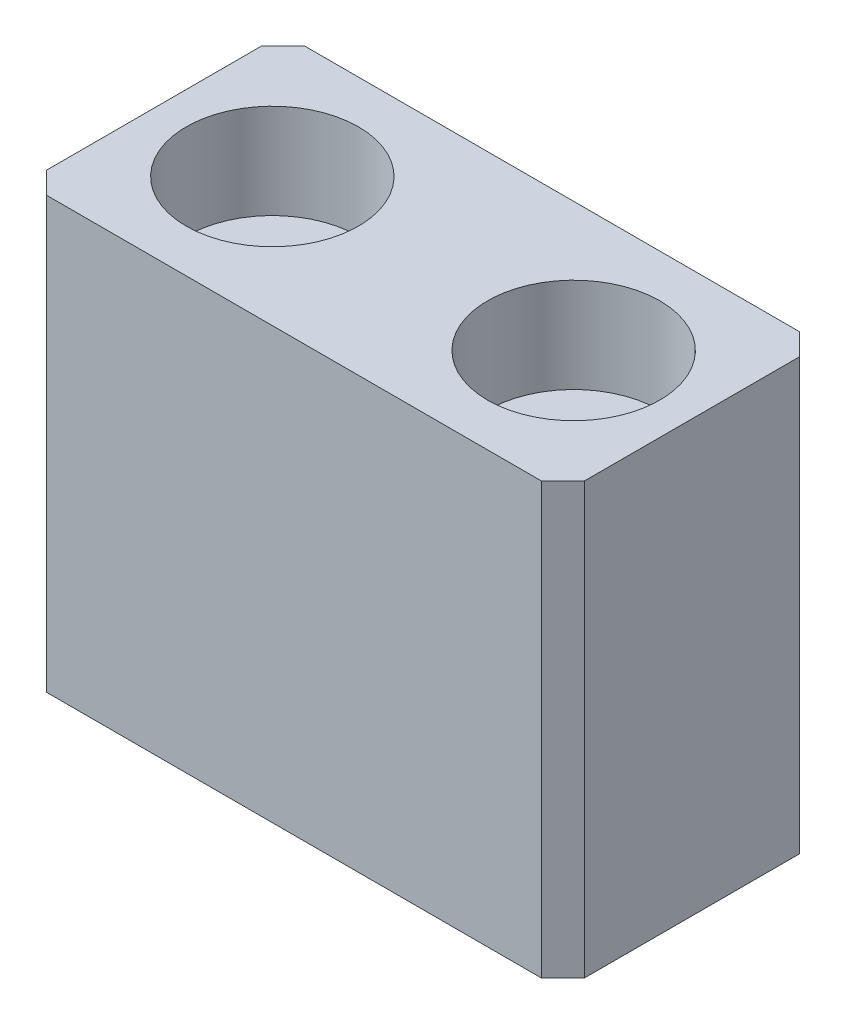
SolidWorks part; units mm, degrees
material "A6063"
ref_plane "Front Plane" through (0, 0, 0) normal (0, 0, 1) x (1, 0, 0)
ref_plane "Top Plane" through (0, 0, 0) normal (0, 1, 0) x (1, 0, 0)
ref_plane "Right Plane" through (0, 0, 0) normal (1, 0, 0) x (0, 0, -1)
sketch "Sketch1" plane through (0, 0, 0) normal (0, 0, 1) x (1, 0, 0)
  line L1 (-12.5, 10) -> (12.5, 10)
  line L2 (-12.5, 10) -> (-12.5, -10)
  line L3 (-12.5, -10) -> (12.5, -10)
  line L4 (12.5, 10) -> (12.5, -10)
  line L5 (-12.5, 10) -> (12.5, -10) construction
  line L6 (-12.5, -10) -> (12.5, 10) construction
  point P0 (0, 0)
  dimension "D1" = 25
  dimension "D2" = 20
extrude "Boss-Extrude1" add sketch "Sketch1" along normal blind 12
hole_wizard "CBORE for M4 Hex Socket Head Cap Screw1" positions "Sketch3" profile "Sketch2" counterbore size "M4" standard "Iso" end condition through all
sketch "Sketch3" plane through (0, 10, 0) normal (0, 1, 0) x (1, 0, 0)
  line L0 (-12.5, -6) -> (-9.7925, -6) construction
  line L1 (-12.5, -12) -> (-12.5, 0) construction
  line L3 (0, 0) -> (0, -7.5271) construction
  point P0 (-7, -6)
  point P14 (7, -6)
  dimension "D1" = 7
sketch "Sketch2" plane through (-7, 10, 6) normal (1, 0, 0) x (0, 0, 1)
  line L0 (0, 0) -> (0, 20)
  line L1 (0, 20) -> (2.25, 20)
  line L3 (2.25, 20) -> (2.25, 4.4)
  line L4 (2.25, 4.4) -> (4, 4.4)
  line L5 (4, 4.4) -> (4, 0)
  line L7 (4, 0) -> (0, 0)
  line L11 (0, -6.35) -> (0, 107.95) construction
  dimension "通孔孔直径" = 4.5
  dimension "通孔孔深度" = 20
  dimension "柱形沉头孔直径" = 8
  dimension "柱形沉头孔深度" = 4.4
chamfer "Chamfer1" distance 1 angle 45 4 edges at (-12.5, 0, 0) (12.5, 0, 0) (12.5, 0, 12) (-12.5, 0, 12)
